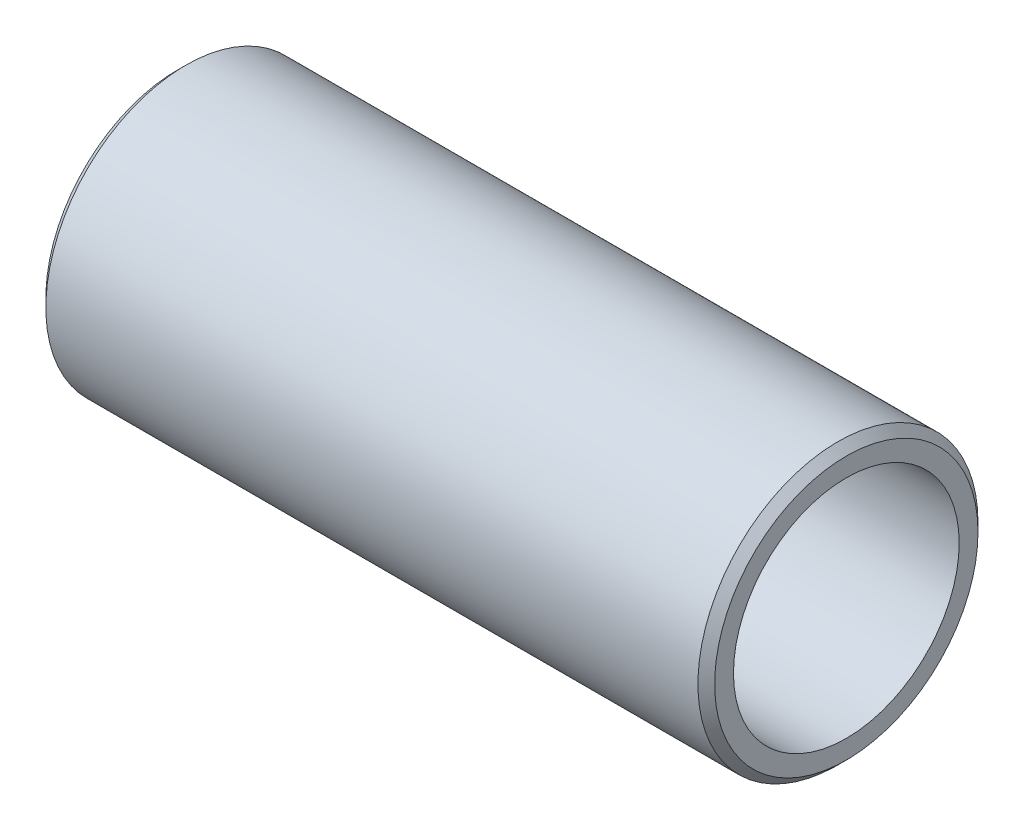
SolidWorks part; units mm, degrees
material "Q235"
ref_plane "前视基准面" through (0, 0, 0) normal (0, 0, 1) x (1, 0, 0)
ref_plane "上视基准面" through (0, 0, 0) normal (0, 1, 0) x (1, 0, 0)
ref_plane "右视基准面" through (0, 0, 0) normal (1, 0, 0) x (0, 0, -1)
sketch "草图1" plane through (0, 0, 0) normal (1, 0, 0) x (0, 0, -1)
  circle A0 centre (0, 0) radius 16.75
  dimension "D1" = 33.5
extrude "拉伸-薄壁1" add sketch "草图1" along normal blind 80 thin thin type one direction reverse wall 3.25
cosmetic thread "装饰螺纹线1" parameters "D1"=20, "D2"=30.291
cosmetic thread "装饰螺纹线2" parameters "D1"=20, "D2"=30.291
chamfer "倒角1" distance 1 angle 45 2 edges at (0, 0, -16.75) (80, 0, -16.75)
